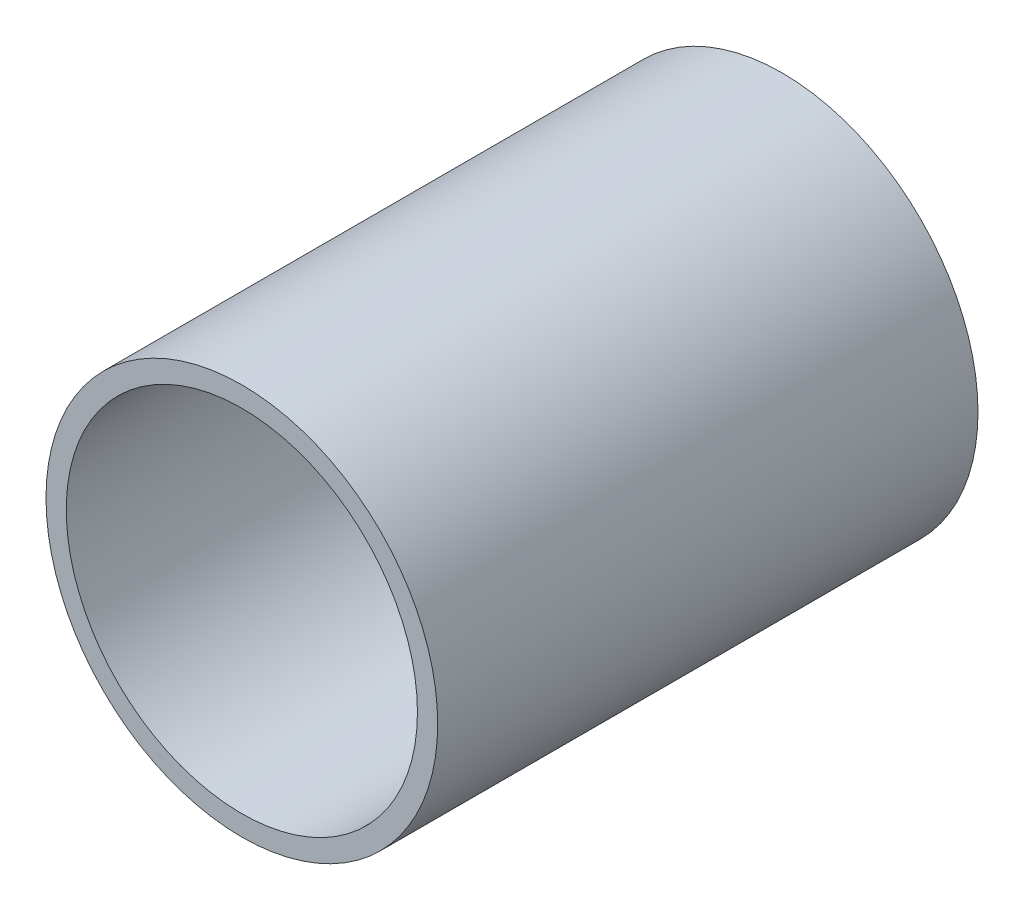
SolidWorks part; units mm, degrees
ref_plane "Front Plane" through (0, 0, 0) normal (0, 0, 1) x (1, 0, 0)
ref_plane "Top Plane" through (0, 0, 0) normal (0, 1, 0) x (1, 0, 0)
ref_plane "Right Plane" through (0, 0, 0) normal (1, 0, 0) x (0, 0, -1)
sketch "Sketch1" plane through (0, 0, 0) normal (0, 0, 1) x (1, 0, 0)
  circle A0 centre (0, 0) radius 3.683
  circle A1 centre (0, 0) radius 3.302
  dimension "D1" = 7.366
  dimension "D2" = 6.604
extrude "Boss-Extrude1" add sketch "Sketch1" along normal blind 10.16
scale "Scale1" bodies to scale 101 scale about origin uniform scaling yes scale factor 2
